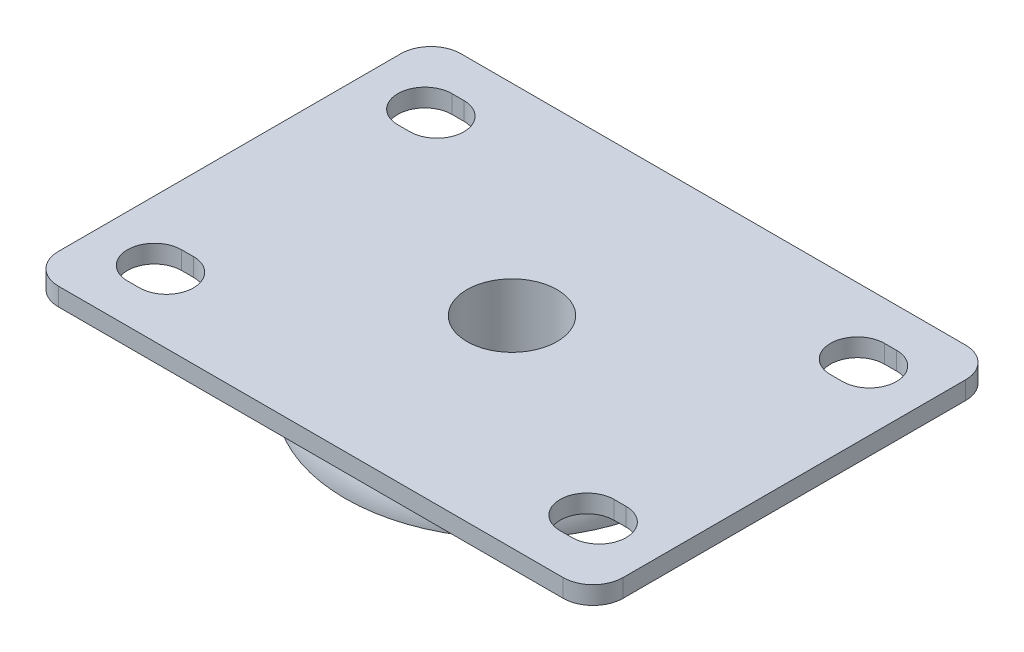
SolidWorks part; units mm, degrees
ref_plane "前视基准面" through (0, 0, 0) normal (0, 0, 1) x (1, 0, 0)
ref_plane "上视基准面" through (0, 0, 0) normal (0, 1, 0) x (1, 0, 0)
ref_plane "右视基准面" through (0, 0, 0) normal (1, 0, 0) x (0, 0, -1)
sketch "草图2" plane through (0, 0, 0) normal (0, 1, 0) x (1, 0, 0)
  line L0 (0, 0) -> (62.8165, 0) construction
  line L1 (0, 0) -> (0, 36.0613) construction
  line L3 (-47, 33.5) -> (47, 33.5)
  line L4 (-47, 33.5) -> (-47, -33.5)
  line L5 (-47, -33.5) -> (47, -33.5)
  line L6 (47, 33.5) -> (47, -33.5)
  dimension "D1" = 67
  dimension "D2" = 94
extrude "拉伸1" add sketch "草图2" along normal blind 3
fillet "圆角1" radius 5 4 edges at (-47, 1.5, -33.5) (-47, 1.5, 33.5) (47, 1.5, -33.5) (47, 1.5, 33.5)
sketch "草图3" plane through (0, 3, 0) normal (0, 1, 0) x (-1, 0, 0)
  line L0 (0, 0) -> (15.4632, 0) construction
  line L1 (0, 0) -> (0, 16.8874) construction
  line L2 (35, 27) -> (37, 27)
  line L3 (35, 18) -> (37, 18)
  line L4 (-35, 18) -> (-37, 18)
  line L5 (-35, 27) -> (-37, 27)
  line L6 (-35, -27) -> (-37, -27)
  line L7 (-35, -18) -> (-37, -18)
  line L8 (35, -18) -> (37, -18)
  line L9 (35, -27) -> (37, -27)
  arc A0 (35, 27) -> (35, 18) centre (35, 22.5) ccw
  arc A1 (37, 18) -> (37, 27) centre (37, 22.5) ccw
  arc A2 (-37, 18) -> (-37, 27) centre (-37, 22.5) cw
  arc A3 (-35, 27) -> (-35, 18) centre (-35, 22.5) cw
  arc A4 (-35, -27) -> (-35, -18) centre (-35, -22.5) ccw
  arc A5 (-37, -18) -> (-37, -27) centre (-37, -22.5) ccw
  arc A6 (37, -18) -> (37, -27) centre (37, -22.5) cw
  arc A7 (35, -27) -> (35, -18) centre (35, -22.5) cw
  dimension "D2" = 11
  dimension "D4" = 61
  dimension "D1" = 9
  dimension "D3" = 36
extrude "切除-拉伸1" cut sketch "草图3" against normal through all
sketch "草图4" plane through (0, 0, 0) normal (0, 0, 1) x (1, 0, 0)
  line L0 (0, 11.0628) -> (0, -9.9618) construction
  line L1 (0, -9.5) -> (27.75, -9.5)
  line L2 (0, -9.5) -> (0, 0)
  line L3 (0, 0) -> (18.25, 0)
  line L4 (-42, 0) -> (42, 0) construction
  arc A0 (18.25, 0) -> (27.75, -9.5) centre (18.25, -9.5) cw
  dimension "D1" = 9.5
  dimension "D2" = 55.5
revolve "旋转1" add sketch "草图4" angle 360 about L0
sketch "草图6" plane through (0, -9.5, 0) normal (0, -1, 0) x (1, 0, 0)
  circle A0 centre (0, 0) radius 7.5
  dimension "D1" = 15
extrude "切除-拉伸2" cut sketch "草图6" against normal through all
